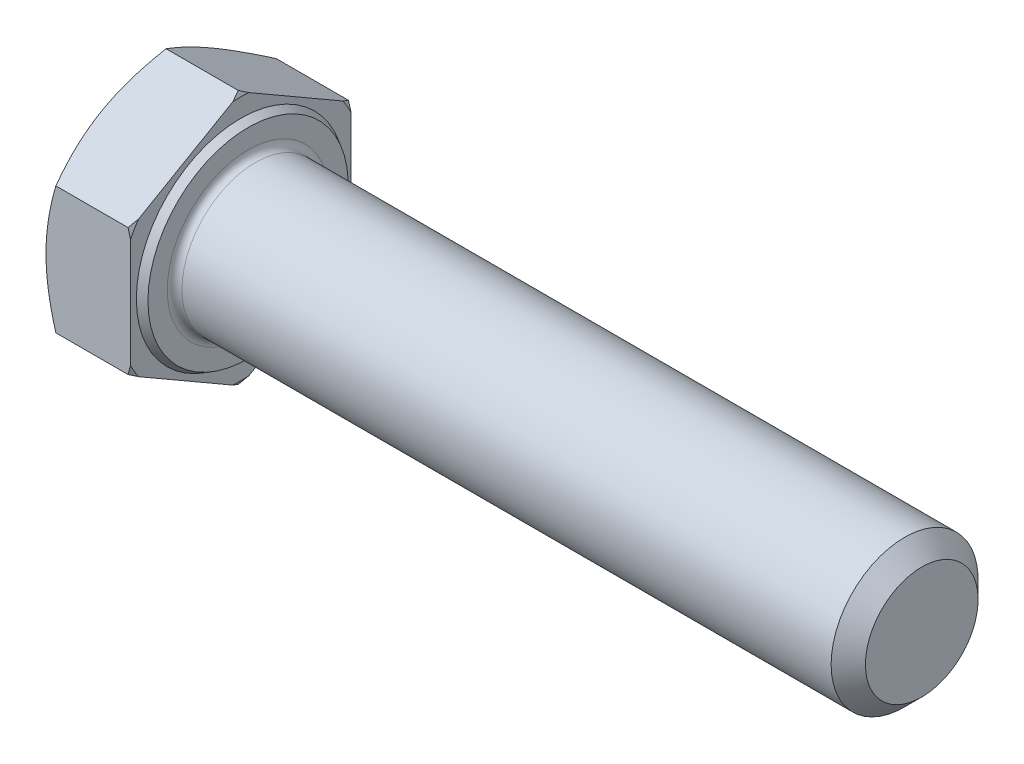
from build123d import *

# Parameters (mm, degrees)
BOSS_EXTRUDE_DEPTH = 7.5
CHAMFER_2_SIZE     = 1.4


with BuildPart() as part:
    # Sketch1 → Boss-Extrude (new body)
    with BuildSketch(Plane(origin=(0, 0, 0), x_dir=(0, 0, -1), z_dir=(1, 0, 0))):
        Polygon((9, 5.196152423), (9, -5.196152423), (0, -10.392304845), (-9, -5.196152423), (-9, 5.196152423), (0, 10.392304845), align=None)
    extrude(amount=BOSS_EXTRUDE_DEPTH)

    # Sketch2 → Boss-Revolve1 (revolve)
    with BuildSketch(Plane.XY, mode=Mode.PRIVATE) as boss_revolve1_sk:
        Polygon((0, 0), (62.5, 0), (62.5, 4.4845), (62.5, 6), (7.5, 6), (0, 6), align=None)
    revolve(boss_revolve1_sk.sketch.rotate(Axis((0, 0, 0), (-1, 0, 0)), 90), axis=Axis((0, 0, 0), (-1, 0, 0)))

    # Sketch3 → Cut-Revolve1 (revolve, cut)
    with BuildSketch(Plane.XY):
        Polygon((0, 9), (3.690598923, 15.392304845), (3.690598923, 20.392304845), (-10, 20.392304845), (-10, 9), align=None)
    revolve(axis=Axis((0, 0, 0), (1, 0, 0)), mode=Mode.SUBTRACT)

    # Sketch5 → Cut-Revolve2 (revolve, cut)
    with BuildSketch(Plane.XY):
        Polygon((7.5, 9), (3.809401077, 15.392304845), (3.809401077, 20.392304845), (13.809401077, 20.392304845), (13.809401077, 9), align=None)
    revolve(axis=Axis((0, 0, 0), (1, 0, 0)), mode=Mode.SUBTRACT)

    # Sketch4 → Cut-Revolve3 (revolve, cut)
    with BuildSketch(Plane.XY, mode=Mode.PRIVATE) as cut_revolve3_sk:
        Polygon((7.5, 8.177264973), (6.9, 8.523675135), (6.9, 20.392304845), (7.5, 20.392304845), align=None)
    revolve(cut_revolve3_sk.sketch.rotate(Axis((0, 0, 0), (1, 0, 0)), 90), axis=Axis((0, 0, 0), (1, 0, 0)), mode=Mode.SUBTRACT)

    # Chamfer 2
    chamfer_2_edges = [part.edges().sort_by_distance(p)[0] for p in [
        (62.5, 0, 6),
    ]]
    chamfer(chamfer_2_edges, length=CHAMFER_2_SIZE)

    # Sketch9 → Revolve1 (revolve)
    with BuildSketch(Plane.XY, mode=Mode.PRIVATE) as revolve1_sk:
        with BuildLine():
            Line((7.5, 6.6), (7.5, 6))
            Line((7.5, 6), (8.1, 6))
            ThreePointArc((8.1, 6), (7.675735931, 6.175735931), (7.5, 6.6))
        make_face()
    revolve(revolve1_sk.sketch.rotate(Axis((0, 0, 0), (1, 0, 0)), 90), axis=Axis((0, 0, 0), (1, 0, 0)))


solid = part.part
